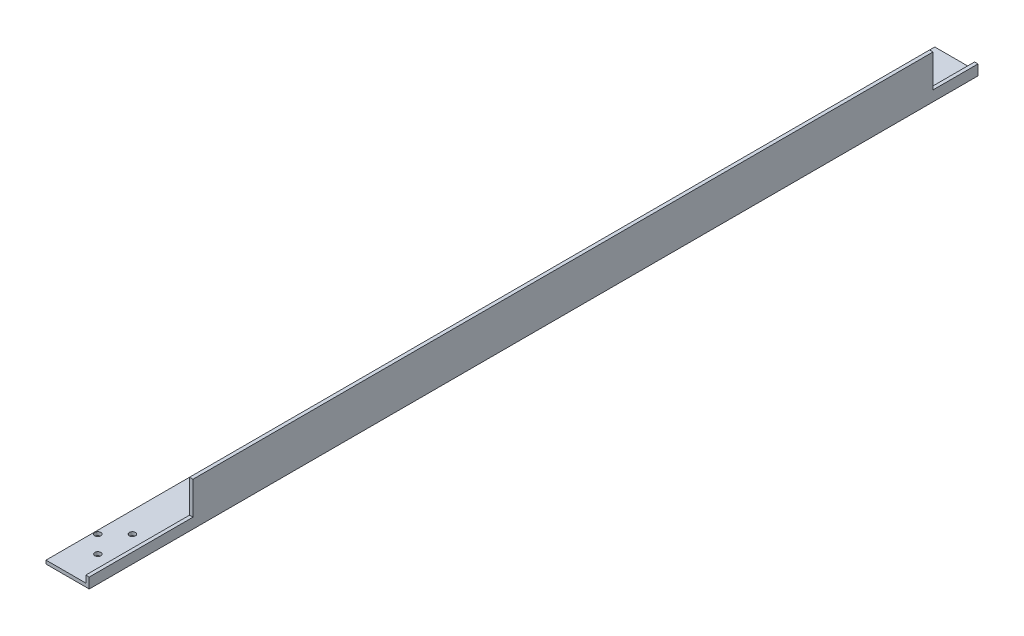
from build123d import *

# Parameters (mm, degrees)
EXTRUDE_1_DEPTH     = 1285
HOLE_WIZARD_M20_1_D = 17.5
SKETCH_4_W          = 300
SKETCH_4_H          = 95
SKETCH_4_W_2        = 130
CUT_EXTRUDE_1_DEPTH = 1297.177071237


with BuildPart() as part:
    # 草图1 → 凸台-拉伸1 (new, symmetric)
    with BuildSketch(Plane.XY):
        Polygon((-125, 0), (0, 0), (0, 125), (-10, 125), (-10, 10), (-125, 10), align=None)
    extrude(amount=EXTRUDE_1_DEPTH, both=True)

    # M20 螺纹孔1 (through all)
    with Locations(Plane(origin=(0, 10, 0), x_dir=(1, 0, 0), z_dir=(0, 1, 0))):
        with Locations((-100, 965), (-50, 965), (-50, 1185), (-100, 1185), (-115, -1145), (-65, -1095), (-65, -1195)):
            Hole(HOLE_WIZARD_M20_1_D / 2)

    # 草图4 → 切除-拉伸1 (cut, through all)
    with BuildSketch(Plane.ZY.offset(10)):
        with Locations((1135, 77.5)):
            Rectangle(SKETCH_4_W, SKETCH_4_H)
        with Locations((-1220, 77.5)):
            Rectangle(SKETCH_4_W_2, SKETCH_4_H)
    extrude(amount=-CUT_EXTRUDE_1_DEPTH, mode=Mode.SUBTRACT)


solid = part.part
